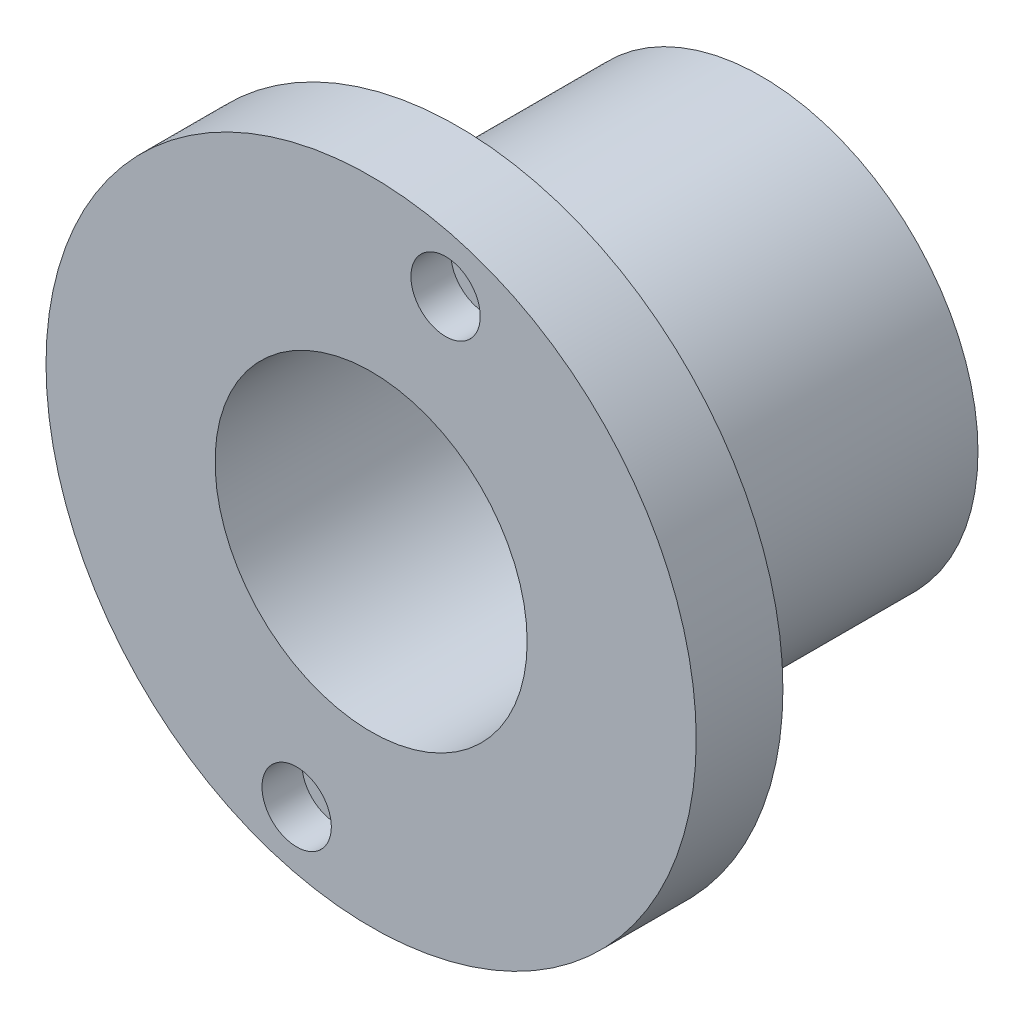
SolidWorks part; units mm, degrees
ref_plane "Front Plane" through (0, 0, 0) normal (0, 0, 1) x (1, 0, 0)
ref_plane "Top Plane" through (0, 0, 0) normal (0, 1, 0) x (1, 0, 0)
ref_plane "Right Plane" through (0, 0, 0) normal (1, 0, 0) x (0, 0, -1)
sketch "Sketch1" plane through (0, 0, 0) normal (0, 0, 1) x (1, 0, 0)
  circle A0 centre (0, 0) radius 18
  circle A1 centre (0, 0) radius 25
  dimension "D1" = 36
  dimension "D2" = 50
extrude "Boss-Extrude1" add sketch "Sketch1" along normal blind 35
sketch "Sketch2" plane through (0, 0, 35) normal (0, 0, 1) x (1, 0, 0)
  circle A0 centre (0, 0) radius 37.5
  circle A1 centre (0, 0) radius 18 construction
  circle A2 centre (0, 0) radius 18
  dimension "D1" = 75
extrude "Boss-Extrude2" add sketch "Sketch2" along normal blind 10
sketch "Sketch3" plane through (0, 0, 45) normal (0, 0, 1) x (1, 0, 0)
  point P0 (-8.5882, -29.7866)
  point P1 (8.5882, 29.7866)
hole_wizard "Hole size per socket head cap screw type3" positions "Sketch4" profile "Sketch5" counterbore size "M4" standard "GB" end condition through all
sketch "Sketch4" plane through (0, 0, 45) normal (0, 0, 1) x (1, 0, 0)
  point P0 (-8.5882, -29.7866)
  point P3 (8.5882, 29.7866)
sketch "Sketch5" plane through (-8.5882, -29.7866, 45) normal (1, 0, 0) x (0, -1, 0)
  line L0 (0, 0) -> (0, 45)
  line L1 (0, 45) -> (2.25, 45)
  line L3 (2.25, 45) -> (2.25, 4.6)
  line L4 (2.25, 4.6) -> (4, 4.6)
  line L5 (4, 4.6) -> (4, 0)
  line L7 (4, 0) -> (0, 0)
  line L11 (0, -6.35) -> (0, 107.95) construction
  dimension "通孔孔直径" = 4.5
  dimension "通孔孔深度" = 45
  dimension "柱形沉头孔直径" = 8
  dimension "柱形沉头孔深度" = 4.6
